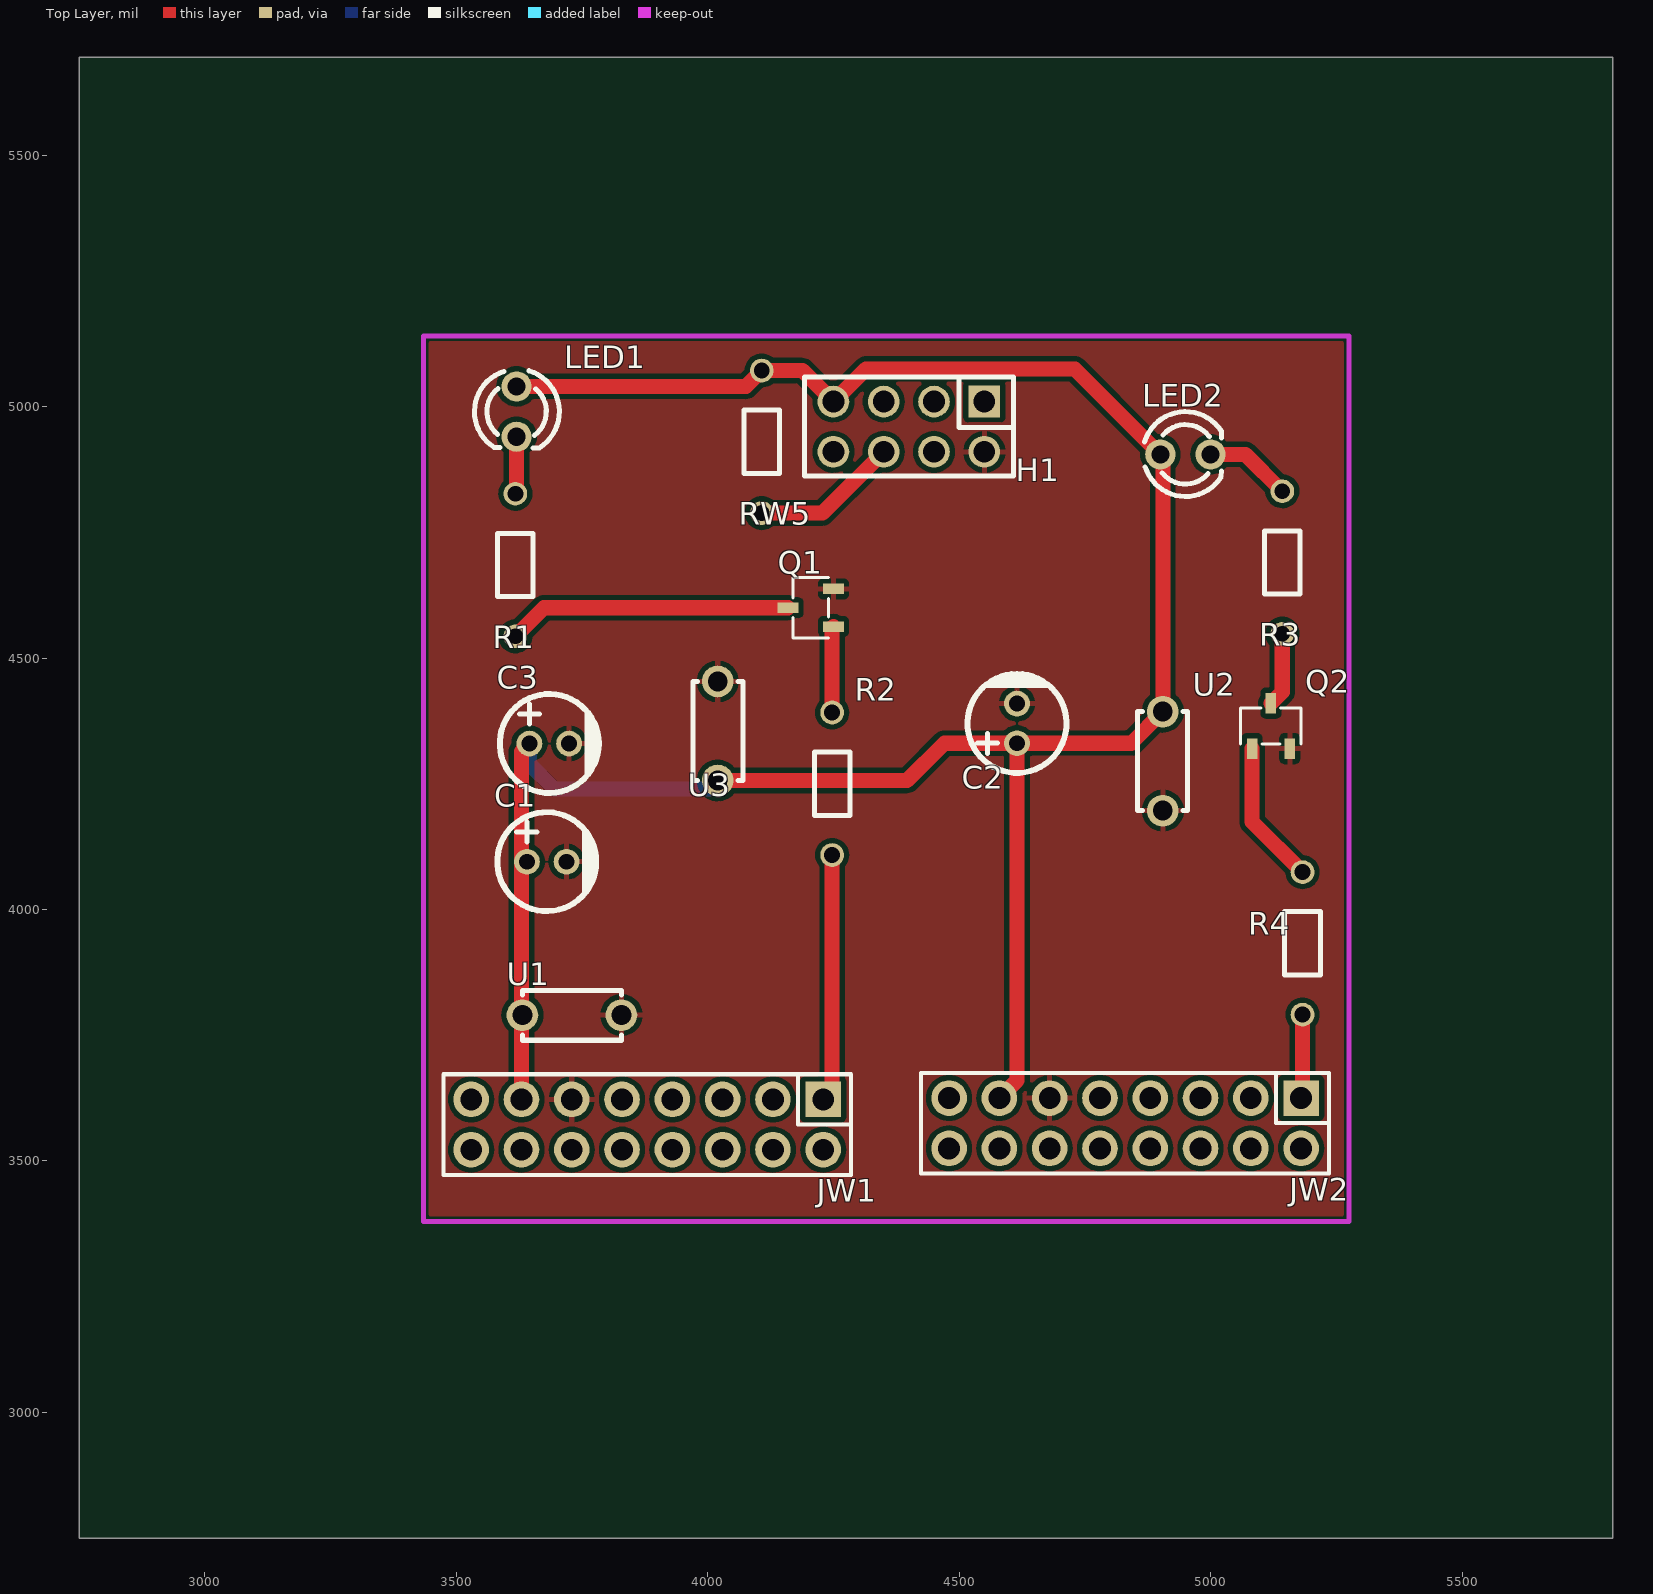
[diagram p0: Top Layer view]
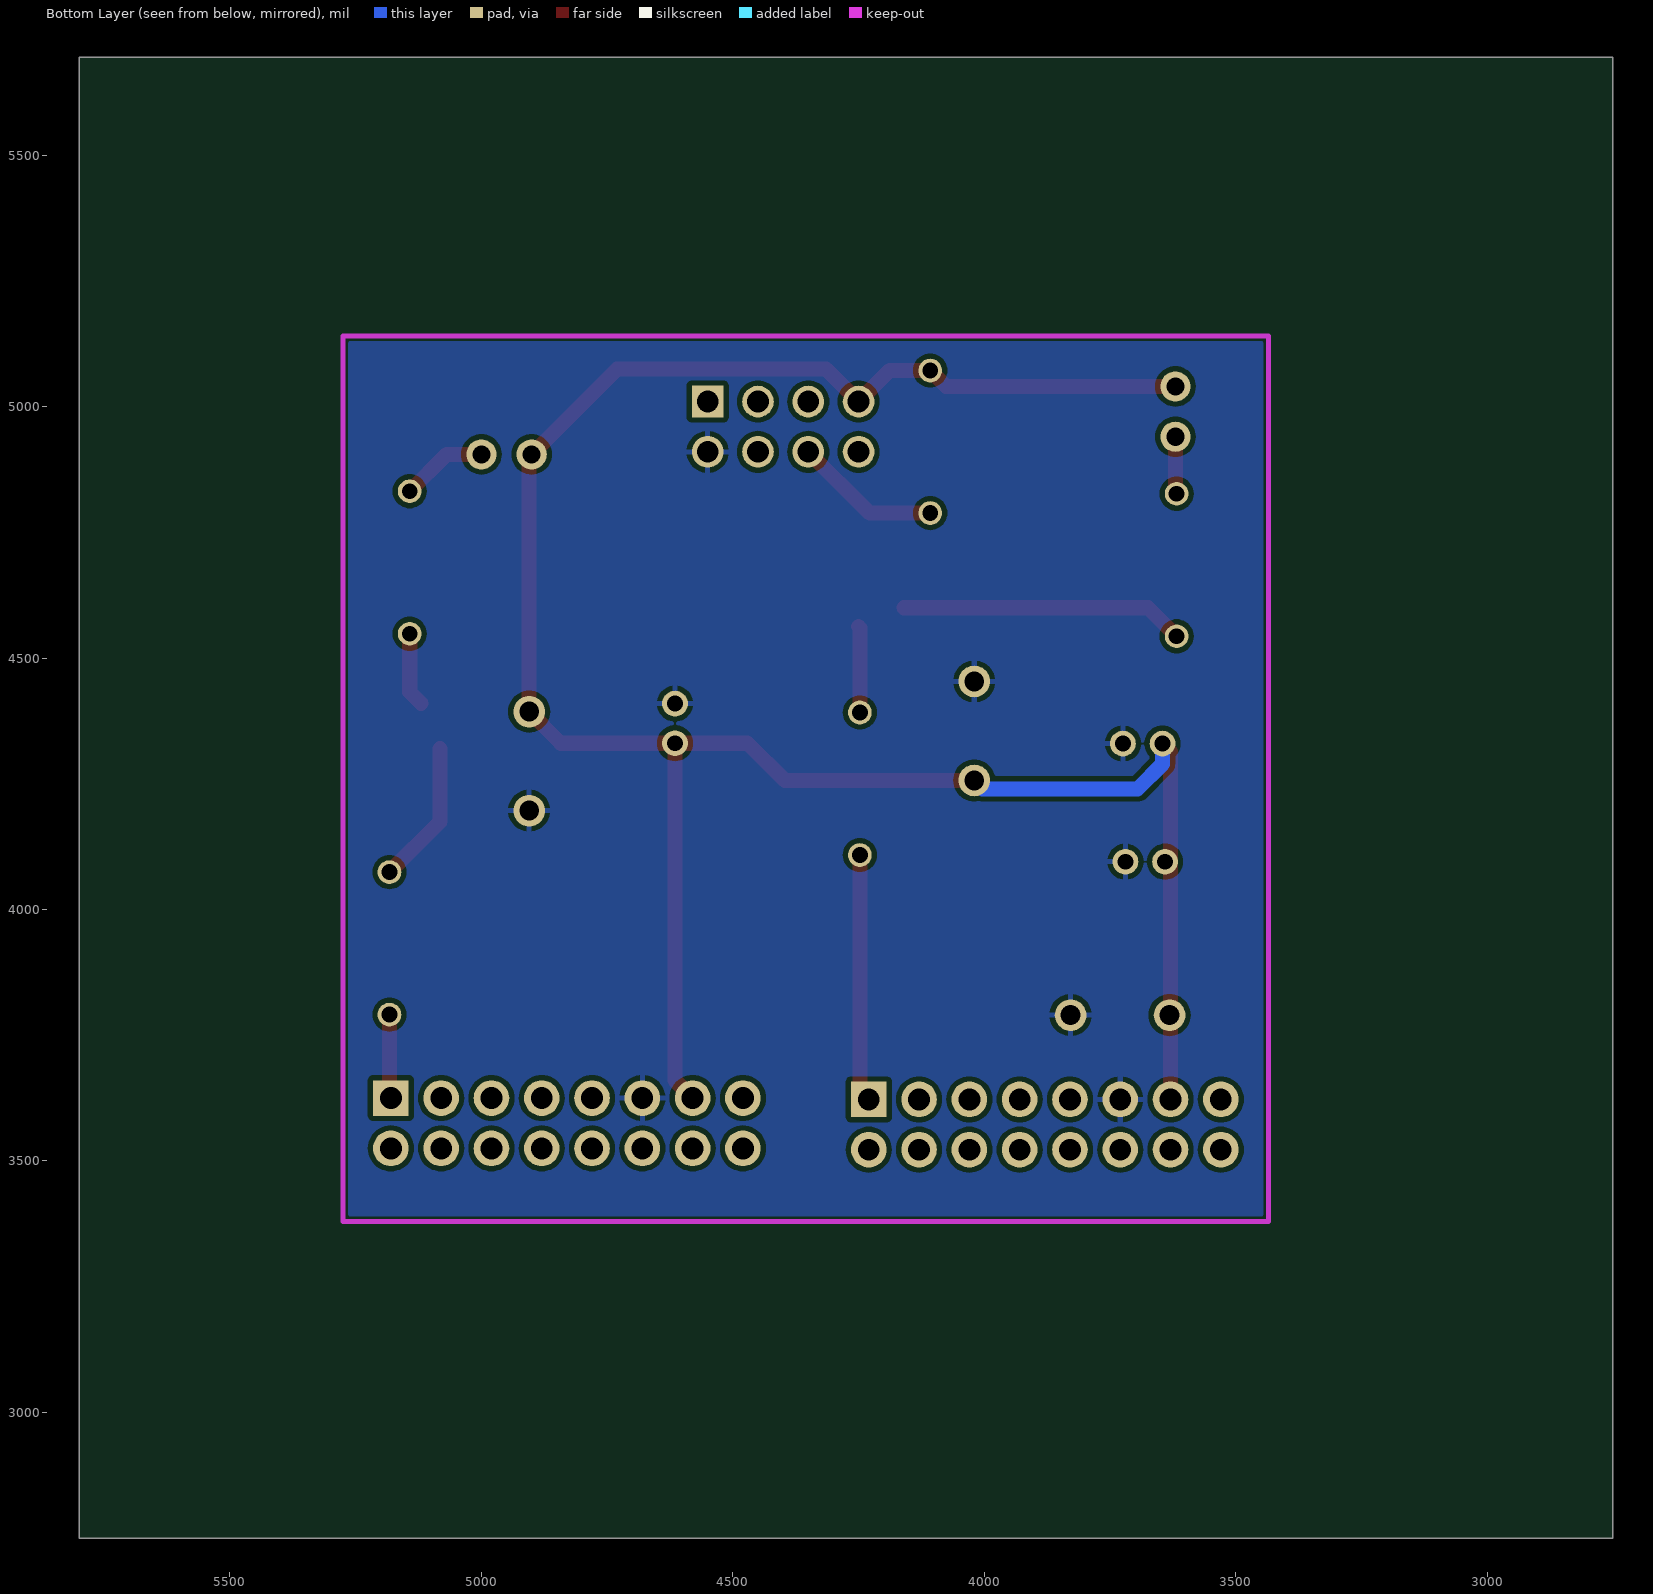
[diagram p1: Bottom Layer view, seen from below]
# Altium PCB MISC49947.pcbdoc
Units mil, origin at the board's own origin, x right, y up, seen from the top; angles counter-clockwise.
Board outline 3050 x 2945 mil, 2 copper layers (Top Layer, Bottom Layer), stack 62.206 mil thick; 18 components, 21 nets, 72 pads, 0 vias.

## Layer stack, top to bottom
Top Solder Mask Layer: solder mask 0.394, Dk 3.3
Top Layer: signal copper 1.379
Dielectric1: surface 59.449, FR4, Dk 4.5
Bottom Layer: signal copper 1.378
Bottom Solder Mask Layer: solder mask 0.394, Dk 3.3

## Board outline
5800,2750 2750,2750 2750,5695 5800,5695

## Design rules (kind name [scope] priority, off if disabled: settings)
BoardOutlineClearance copperThickness2oz_1 [All] p2 off: genericclearance=7.99 ignorepadtopadclearanceinfootprint=FALSE except(0: Arc-SplitContinuation Track-SplitContinuation SMDPad-SplitContinuation THPad-SplitContinuation Via-SplitContinuation Fill-SplitContinuation Region-SplitContinuation Poly-SplitContinuation Text-SplitContinuation Hole-SplitContinuation; 5.98: Arc-CutoutEdge SMDPad-CutoutEdge THPad-CutoutEdge Via-CutoutEdge Fill-CutoutEdge Region-CutoutEdge Text-CutoutEdge; 6.93: Hole-OutlineEdge Hole-CutoutEdge; 10: Poly-OutlineEdge Poly-CutoutEdge; 11.81: Arc-OutlineEdge Track-OutlineEdge SMDPad-OutlineEdge THPad-OutlineEdge Via-OutlineEdge Fill-OutlineEdge Region-OutlineEdge Text-OutlineEdge Track-CutoutEdge)
BoardOutlineClearance copperThickness1oz_1 [All] p4: genericclearance=4.02 ignorepadtopadclearanceinfootprint=FALSE except(0: Arc-SplitContinuation Track-SplitContinuation SMDPad-SplitContinuation THPad-SplitContinuation Via-SplitContinuation Fill-SplitContinuation Region-SplitContinuation Poly-SplitContinuation Text-SplitContinuation Hole-SplitContinuation; 6: SMDPad-CutoutEdge THPad-CutoutEdge Via-CutoutEdge Fill-CutoutEdge Region-CutoutEdge Text-CutoutEdge; 6.93: Hole-OutlineEdge Hole-CutoutEdge; 10: Poly-OutlineEdge Poly-CutoutEdge; 11.8: Arc-OutlineEdge Track-OutlineEdge SMDPad-OutlineEdge THPad-OutlineEdge Via-OutlineEdge Fill-OutlineEdge Region-OutlineEdge Text-OutlineEdge; 11.81: Arc-CutoutEdge Track-CutoutEdge)
Clearance copperThickness2oz [All] p1 off: gap=7.99 ignorepadtopadclearanceinfootprint=FALSE except(5.98: SMDPad-Track SMDPad-SMDPad THPad-Track SMDPad-THPad THPad-THPad Track-Via SMDPad-Via THPad-Via Via-Via Fill-Track Region-Track Fill-SMDPad Region-SMDPad Fill-THPad Region-THPad Fill-Via Region-Via Fill-Fill Fill-Region Region-Region Arc-Track Arc-SMDPad Arc-THPad Arc-Via Fill-Arc Region-Arc Arc-Arc Text-Track SMDPad-Text Text-THPad Text-Via Fill-Text Region-Text Arc-Text Text-Text; 6.93: Hole-Track Hole-SMDPad Hole-THPad Hole-Via Fill-Hole Region-Hole Hole-Arc Hole-Text; 10: Poly-Track Poly-SMDPad Poly-THPad Poly-Via Poly-Fill Poly-Region Poly-Poly Poly-Arc Poly-Text Poly-Hole)
Clearance copperThickness1oz [All] p3: gap=4.02 ignorepadtopadclearanceinfootprint=FALSE except(5.98: SMDPad-Track SMDPad-SMDPad THPad-Track SMDPad-THPad THPad-THPad Track-Via SMDPad-Via THPad-Via Via-Via Fill-Track Region-Track Fill-SMDPad Region-SMDPad Fill-THPad Region-THPad Fill-Via Region-Via Fill-Fill Fill-Region Region-Region; 6: Arc-Track Arc-SMDPad Arc-THPad Arc-Via Fill-Arc Region-Arc Arc-Arc Text-Track SMDPad-Text Text-THPad Text-Via Fill-Text Region-Text Arc-Text Text-Text; 6.93: Hole-Track Hole-SMDPad Hole-THPad Hole-Via Fill-Hole Region-Hole Hole-Arc Hole-Text; 10: Poly-Track Poly-SMDPad Poly-THPad Poly-Via Poly-Fill Poly-Region Poly-Poly Poly-Arc Poly-Text Poly-Hole)
Creepage creepage [All] p1: checkdistance=0 ignoreinternallayers=TRUE applytopolygonpour=TRUE
DiffPairsRouting differentialPair [All] p1: maxlimit=6 minlimit=6 mostfreqgap=6 toplayer_minwidth=5 toplayer_prefwidth=10 toplayer_maxwidth=100 toplayer_mingap=6 toplayer_prefgap=6 toplayer_maxgap=6 bottomlayer_minwidth=5 bottomlayer_prefwidth=10 bottomlayer_maxwidth=100 bottomlayer_mingap=6 bottomlayer_prefgap=6 bottomlayer_maxgap=6 maxuncoupledlength=10
HoleToHoleClearance otherClearance [All] p1: gap=11.81 allowstackedmicrovias=TRUE
Length netLength [All] p1: minlimit=0 maxlimit=0
MatchedLengths netLengthTolerance [All] p1: tolerance=1000
PasteMaskExpansion pasteMaskExpansion [All] p1: expansion=0
PlaneConnect innerPlane [All] p1: planeconnectstyle=Relief reliefexpansion=20 reliefentries=4 reliefconductorwidth=10 reliefairgap=10
PolygonConnect copperRegion [All] p1: connectstyle=Relief reliefconductorwidth=10 reliefentries=4 polygonreliefangle="90 Angle" airgapwidth=10 via.connectstyle=Relief via.reliefconductorwidth=10 via.reliefentries=4 via.polygonreliefangle="90 Angle" via.airgapwidth=10
RoutingVias viaSize [All] p1: holewidth=12.01 width=24.02 viastyle="Through Hole" minholewidth=11.81 minwidth=19.68 maxholewidth=248.03 maxwidth=393.7
SolderMaskExpansion solderMaskExpansion [IsVia] p1: expansion=-1000 istentingtop=TRUE
SolderMaskExpansion solderMaskExpansion [All] p2: expansion=2 istentingtop=FALSE
Width copperThickness2oz_2 [All] p1 off: maxlimit=100 minlimit=8 preferedwidth=10
Width copperThickness1oz_2 [All] p2: maxlimit=100 minlimit=5 preferedwidth=10

## Components (designator, comment, footprint, x,y, rotation, side; value= is the part's Value field where it differs from the comment)
C1 "10uF" CAP-TH_BD5.0-P2.00-D0.8-FD-10UF50VC110GL 3680,4095 r0 top
C2 "10uF" CAP-TH_BD5.0-P2.00-D0.8-FD-10UF50VC110GL 4615,4370 r90 top
C3 "10uF" CAP-TH_BD5.0-P2.00-D0.8-FD-10UF50VC110GL 3685,4330 r0 top
H1 "" HDR-TH_8P-P2.54-V-F-R2-C4-S2.54-1 4400,4960 r180 top
JW1 "" HDR-TH_16P-P2.54-V-F-R2-C8-S2.54-1 3879.69,3572.38 r180 top
JW2 "" HDR-TH_16P-P2.54-V-F-R2-C8-S2.54-1 4830,3575 r180 top
LED1 "" LED_TH-3mm 3620,4990 r270 top
LED2 "" LED_TH-3mm 4950,4905 r0 top
Q1 "2SC2412KT146Q" SOT-346_L2.9-W1.6-P1.90-LS2.8-TR-CW-1 4205,4600 r0 top
Q2 "2SC2412KT146Q" SOT-346_L2.9-W1.6-P1.90-LS2.8-TR-CW-1 5120,4365 r270 top
R1 "100Ω" Res_1/8W 3620,4685 r90 top
R2 "100Ω" Res_1/8W 4245,4250 r270 top
R3 "100Ω" Res_1/8W 5145,4690 r90 top
R4 "100Ω" Res_1/8W 5180.31,3932.62 r270 top
RW5 "4.7kΩ" Res_1/8W 4110,4930 r90 top
U1 "100nF" CAP-TH_L5.0-W2.5-P5.00-D1.0 3730,3790 r0 top
U2 "100nF" CAP-TH_L5.0-W2.5-P5.00-D1.0 4905,4295 r270 top
U3 "100nF" CAP-TH_L5.0-W2.5-P5.00-D1.0 4020,4355 r90 top

## Footprints (in the part's own frame and the unit in brackets; to place one, negate y for a bottom-side part, rotate by r counter-clockwise, add the part's x,y. Pads: shape width x height; smd on the part's side, far side on the other; paste and mask are expansions set on the pad)
CAP-TH_BD5.0-P2.00-D0.8-FD-10UF50VC110GL [mm]
  round 1.3 hole 0.8: 1(-1,0) 2(1,0)
  silkscreen extent -2.5,-2.5 2.5,2.5
CAP-TH_L5.0-W2.5-P5.00-D1.0 [mm]
  round 1.6 hole 1: 1(-2.5,0) 2(2.5,0)
  silkscreen extent -2.5,-1.27 2.5,1.25
HDR-TH_8P-P2.54-V-F-R2-C4-S2.54-1 [mm]
  rect 1.6x1.6 hole 1.1: 1(-3.81,-1.27)
  round 1.6 hole 1.1: 2(-3.81,1.27) 3(-1.27,-1.27) 4(-1.27,1.27) 5(1.27,-1.27) 6(1.27,1.27) 7(3.81,-1.27) 8(3.81,1.27)
  silkscreen extent -5.28,-2.5 5.28,2.5
HDR-TH_16P-P2.54-V-F-R2-C8-S2.54-1 [mm]
  rect 1.8x1.8 hole 1.1: 1(-8.89,-1.27)
  round 1.8 hole 1.1: 2(-8.89,1.27) 3(-6.35,-1.27) 4(-6.35,1.27) 5(-3.81,-1.27) 6(-3.81,1.27) 7(-1.27,-1.27) 8(-1.27,1.27) 9(1.27,-1.27) 10(1.27,1.27) 11(3.81,-1.27) 12(3.81,1.27) 13(6.35,-1.27) 14(6.35,1.27) 15(8.89,-1.27) 16(8.89,1.27)
  silkscreen extent -10.3,-2.54 10.3,2.54
LED_TH-3mm [mil]
  round 60 hole 36 paste+0 mask+2: 1(-50,0) 2(50,0)
  silkscreen extent -81,-84 72,85
Res_1/8W [mil]
  round 47.2 hole 31.5 paste+0 mask+2: 1(-141.7,2.48) 2(141.7,2.48)
  silkscreen extent -63,-33 63,38
SOT-346_L2.9-W1.6-P1.90-LS2.8-TR-CW-1 [mm]
  rect 1.045x0.532 smd: 1(1.148,0.95) 2(1.148,-0.95) 3(-1.148,0)
  silkscreen extent -0.9,-1.53 0.9,1.53

## Nets (pads, with @x,y where several pads share a name; then routed paths per layer and width w, separated by ;. In a path a pad name is that pad's centre, name@x,y a point inside that pad or via, vN(x,y) a via of type N, cw(c..) or ccw(c..) an arc to the next point about the centre after c; other vN are vias at no path point)
$1N3: H1.6 RW5.1 | length 292.9
  Top Layer w30: RW5.1 4228.3,4788.3 H1.6
$1N13: Q2.2 R4.1 | length 287
  Top Layer w30: Q2.2 5082.6,4174.51 R4.1
$1N14: Q1.2 R2.1 | length 172
  Top Layer w30: R2.1 4247.48,4559.9 Q1.2
$1N15: Q1.3 R1.1 | length 565.8
  Top Layer w30: R1.1 3674.22,4600 Q1.3
$1N16: Q2.3 R3.1 | length 147.4
  Top Layer w30: Q2.3 5142.52,4432.7 R3.1
$1N40: LED1.2 R1.2 | length 114.3
  Top Layer w30: R1.2 3620,4829.18 LED1.2
$1N42: LED2.2 R3.2 | length 172.9
  Top Layer w30: LED2.2 5069.22,4905 R3.2
+3.3V: C1.1 C2.1 C3.1 H1.7 JW1.13 JW2.13 LED1.1 LED2.1 RW5.2 U1.1 U2.1 U3.1 | length 4748
  Top Layer w30: LED1.1 4075.82,5040 RW5.2 4188.3,5071.7 H1.7 4315,5075 4730,5075 LED2.1 4905,4900 U2.1 4842.2,4330.63 C2.1 ; JW1.13 3629.69,4314.06 C3.1 ; U3.1 4396.57,4256.57 4470.63,4330.63 C2.1 ; JW2.13 4615,3660 C2.1
  Bottom Layer w30: C3.1 3645.63,4289.37 3695,4240 4003.43,4240 U3.1
BAT3V: H1.8
GND: C1.2 C2.2 C3.2 H1.2 JW1.11 JW2.11 Q1.1 Q2.1 U1.2 U2.2 U3.2
PPS: H1.4
RXD1: JW1.7
RXD2: JW2.7
RXD3: H1.1
STATE_LED1: JW1.1 R2.2 | length 493.3
  Top Layer w30: JW1.1 4247.48,3640.17 R2.2
STATE_LED2: JW2.1 R4.2 | length 167.1
  Top Layer w30: JW2.1 5182.79,3627.79 R4.2
TXD1: JW1.5
TXD2: JW2.5
TXD3: H1.3
WIR_RST1: JW1.9
WIR_RST2: JW2.9
pads on no net: H1.5 JW1.2 JW1.3 JW1.4 JW1.6 JW1.8 JW1.10 JW1.12 JW1.14 JW1.15 JW1.16 JW2.2 JW2.3 JW2.4 JW2.6 JW2.8 JW2.10 JW2.12 JW2.14 JW2.15 JW2.16

## Polygon pours and split planes (outlines as drawn)
GND on Top Layer (solid, remove dead copper, pour order 0): 3000,5445 3000,3000 5510,3000 5510,5445
GND on Bottom Layer (solid, remove dead copper, pour order 2): 3035,5220 3035,3100 5550,3100 5550,5220

## Keep-outs
Board Outline Layer:
  lines w10: 3435,3380 5275,3380 5275,5140 3435,5140 3435,3380